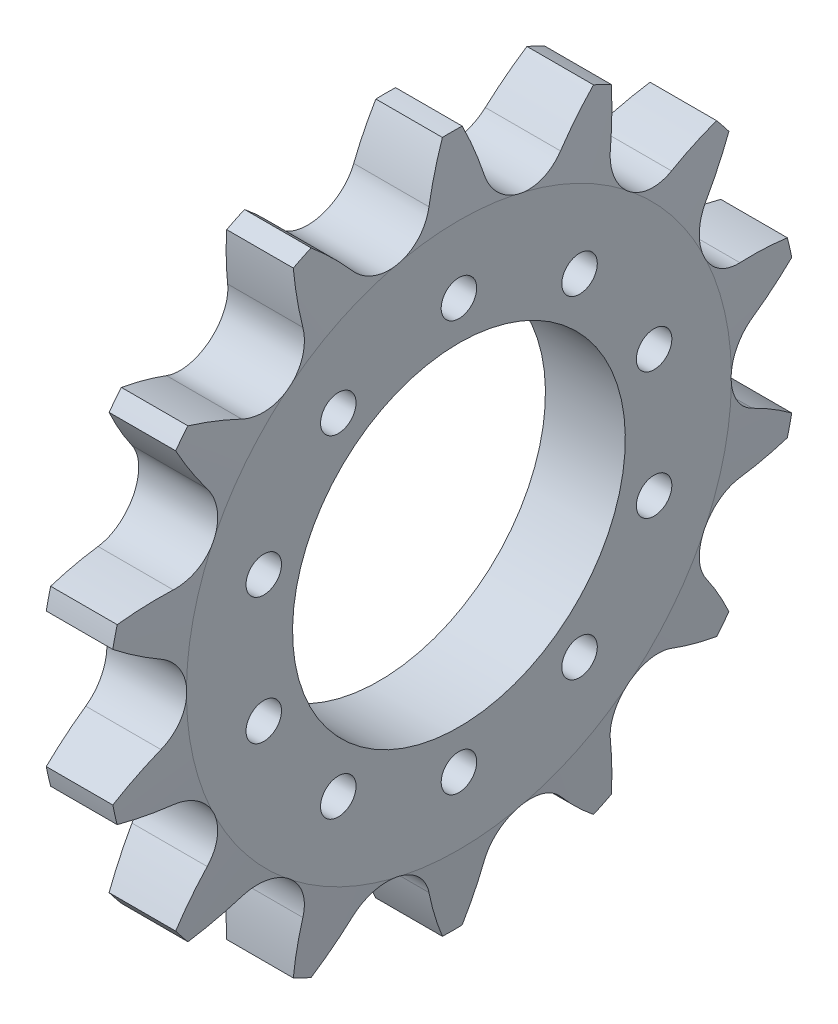
from build123d import *

# Parameters (mm, degrees)
CUT_EXTRUDE1_DEPTH      = 222.350400948
CUT_EXTRUDE1_DEPTH_BACK = 222.350400948
SKETCH3_R               = 196.104739579
SKETCH4_R               = 8
CUT_EXTRUDE2_DEPTH      = 220.258511792
CIRPATTERN1_COUNT       = 10


with BuildPart() as part:
    # Sketch1 → Revolve1 (revolve)
    with BuildSketch(Plane.XY):
        Polygon((15, 156), (-15, 156), (-18, 122.845), (-18, 75), (18, 75), (18, 122.845), align=None)
    revolve(axis=Axis((0, 0, 0), (-1, 0, 0)))

    # Sketch3 → Cut-Extrude1 (cut, two sides: drawn at the far end of the back side and taken through both)
    with BuildSketch(Plane(origin=(0, 0, 0), x_dir=(0, 0, -1), z_dir=(1, 0, 0)).offset(-CUT_EXTRUDE1_DEPTH_BACK)):
        Circle(SKETCH3_R)
        with BuildLine():
            ThreePointArc((153.680060031, 30.870724787), (152.819950235, 34.880156398), (151.855255205, 38.865717112))
            ThreePointArc((151.855255205, 38.865717112), (139.850282677, 40.911426465), (127.715462133, 41.936327702))
            ThreePointArc((127.715462133, 41.936327702), (110.544375247, 53.235365371), (112.416429436, 73.705096444))
            ThreePointArc((112.416429436, 73.705096444), (119.181066239, 83.831496648), (125.066644206, 94.492841037))
            ThreePointArc((125.066644206, 94.492841037), (122.552084877, 97.732026441), (119.953654703, 100.904327079))
            ThreePointArc((119.953654703, 100.904327079), (108.249948172, 97.538685151), (96.872164664, 93.196987947))
            ThreePointArc((96.872164664, 93.196987947), (76.499081239, 95.926813741), (69.304260326, 115.181658044))
            ThreePointArc((69.304260326, 115.181658044), (71.005307103, 127.240295282), (71.682245653, 139.39949124))
            ThreePointArc((71.682245653, 139.39949124), (68.011276107, 141.226870044), (64.293761753, 142.957597559))
            ThreePointArc((64.293761753, 142.957597559), (55.209383833, 134.847211009), (46.842146923, 125.998841744))
            ThreePointArc((46.842146923, 125.998841744), (27.302205992, 119.618780185), (12.465532497, 133.845079658))
            ThreePointArc((12.465532497, 133.845079658), (8.766076073, 145.447592935), (4.100299225, 156.696362581))
            ThreePointArc((4.100299225, 156.696362581), (0, 156.75), (-4.100299225, 156.696362581))
            ThreePointArc((-4.100299225, 156.696362581), (-8.766076073, 145.447592935), (-12.465532497, 133.845079658))
            ThreePointArc((-12.465532497, 133.845079658), (-27.302205992, 119.618780185), (-46.842146923, 125.998841744))
            ThreePointArc((-46.842146923, 125.998841744), (-55.209383833, 134.847211009), (-64.293761753, 142.957597559))
            ThreePointArc((-64.293761753, 142.957597559), (-68.011276107, 141.226870044), (-71.682245653, 139.39949124))
            ThreePointArc((-71.682245653, 139.39949124), (-71.005307103, 127.240295282), (-69.304260326, 115.181658044))
            ThreePointArc((-69.304260326, 115.181658044), (-76.499081239, 95.926813741), (-96.872164664, 93.196987947))
            ThreePointArc((-96.872164664, 93.196987947), (-108.249948172, 97.538685151), (-119.953654703, 100.904327079))
            ThreePointArc((-119.953654703, 100.904327079), (-122.552084877, 97.732026441), (-125.066644206, 94.492841037))
            ThreePointArc((-125.066644206, 94.492841037), (-119.181066239, 83.831496648), (-112.416429436, 73.705096444))
            ThreePointArc((-112.416429436, 73.705096444), (-110.544375247, 53.235365371), (-127.715462133, 41.936327702))
            ThreePointArc((-127.715462133, 41.936327702), (-139.850282677, 40.911426465), (-151.855255205, 38.865717112))
            ThreePointArc((-151.855255205, 38.865717112), (-152.819950235, 34.880156398), (-153.680060031, 30.870724787))
            ThreePointArc((-153.680060031, 30.870724787), (-143.751553546, 23.818841978), (-133.263146, 17.63033656))
            ThreePointArc((-133.263146, 17.63033656), (-122.695, 0), (-133.263146, -17.63033656))
            ThreePointArc((-133.263146, -17.63033656), (-143.751553546, -23.818841978), (-153.680060031, -30.870724787))
            ThreePointArc((-153.680060031, -30.870724787), (-152.819950235, -34.880156398), (-151.855255205, -38.865717112))
            ThreePointArc((-151.855255205, -38.865717112), (-139.850282677, -40.911426465), (-127.715462133, -41.936327702))
            ThreePointArc((-127.715462133, -41.936327702), (-110.544375247, -53.235365371), (-112.416429436, -73.705096444))
            ThreePointArc((-112.416429436, -73.705096444), (-119.181066239, -83.831496648), (-125.066644206, -94.492841037))
            ThreePointArc((-125.066644206, -94.492841037), (-122.552084877, -97.732026441), (-119.953654703, -100.904327079))
            ThreePointArc((-119.953654703, -100.904327079), (-108.249948172, -97.538685151), (-96.872164664, -93.196987947))
            ThreePointArc((-96.872164664, -93.196987947), (-76.499081239, -95.926813741), (-69.304260326, -115.181658044))
            ThreePointArc((-69.304260326, -115.181658044), (-71.005307103, -127.240295282), (-71.682245653, -139.39949124))
            ThreePointArc((-71.682245653, -139.39949124), (-68.011276107, -141.226870044), (-64.293761753, -142.957597559))
            ThreePointArc((-64.293761753, -142.957597559), (-55.209383833, -134.847211009), (-46.842146923, -125.998841744))
            ThreePointArc((-46.842146923, -125.998841744), (-27.302205992, -119.618780185), (-12.465532497, -133.845079658))
            ThreePointArc((-12.465532497, -133.845079658), (-8.766076073, -145.447592935), (-4.100299225, -156.696362581))
            ThreePointArc((-4.100299225, -156.696362581), (0, -156.75), (4.100299225, -156.696362581))
            ThreePointArc((4.100299225, -156.696362581), (8.766076073, -145.447592935), (12.465532497, -133.845079658))
            ThreePointArc((12.465532497, -133.845079658), (27.302205992, -119.618780185), (46.842146923, -125.998841744))
            ThreePointArc((46.842146923, -125.998841744), (55.209383833, -134.847211009), (64.293761753, -142.957597559))
            ThreePointArc((64.293761753, -142.957597559), (68.011276107, -141.226870044), (71.682245653, -139.39949124))
            ThreePointArc((71.682245653, -139.39949124), (71.005307103, -127.240295282), (69.304260326, -115.181658044))
            ThreePointArc((69.304260326, -115.181658044), (76.499081239, -95.926813741), (96.872164664, -93.196987947))
            ThreePointArc((96.872164664, -93.196987947), (108.249948172, -97.538685151), (119.953654703, -100.904327079))
            ThreePointArc((119.953654703, -100.904327079), (122.552084877, -97.732026441), (125.066644206, -94.492841037))
            ThreePointArc((125.066644206, -94.492841037), (119.181066239, -83.831496648), (112.416429436, -73.705096444))
            ThreePointArc((112.416429436, -73.705096444), (110.544375247, -53.235365371), (127.715462133, -41.936327702))
            ThreePointArc((127.715462133, -41.936327702), (139.850282677, -40.911426465), (151.855255205, -38.865717112))
            ThreePointArc((151.855255205, -38.865717112), (152.819950235, -34.880156398), (153.680060031, -30.870724787))
            ThreePointArc((153.680060031, -30.870724787), (143.751553546, -23.818841978), (133.263146, -17.63033656))
            ThreePointArc((133.263146, -17.63033656), (122.695, 0), (133.263146, 17.63033656))
            ThreePointArc((133.263146, 17.63033656), (143.751553546, 23.818841978), (153.680060031, 30.870724787))
        make_face(mode=Mode.SUBTRACT)
    extrude(amount=CUT_EXTRUDE1_DEPTH + CUT_EXTRUDE1_DEPTH_BACK, mode=Mode.SUBTRACT)

    # Sketch4 → Cut-Extrude2 (cut, symmetric)
    with BuildSketch(Plane(origin=(0, 0, 0), x_dir=(0, 0, -1), z_dir=(1, 0, 0))):
        with Locations((0, 92.5)):
            Circle(SKETCH4_R)
    cut_extrude2 = extrude(amount=CUT_EXTRUDE2_DEPTH, both=True, mode=Mode.SUBTRACT)

    # CirPattern1: Cut-Extrude2 ×10 about axis
    cirpattern1_axis = Axis((0, 0, 0), (1, 0, 0))
    for i in range(1, CIRPATTERN1_COUNT):
        add(cut_extrude2.rotate(cirpattern1_axis, i * 360 / CIRPATTERN1_COUNT), mode=Mode.SUBTRACT)


solid = part.part
